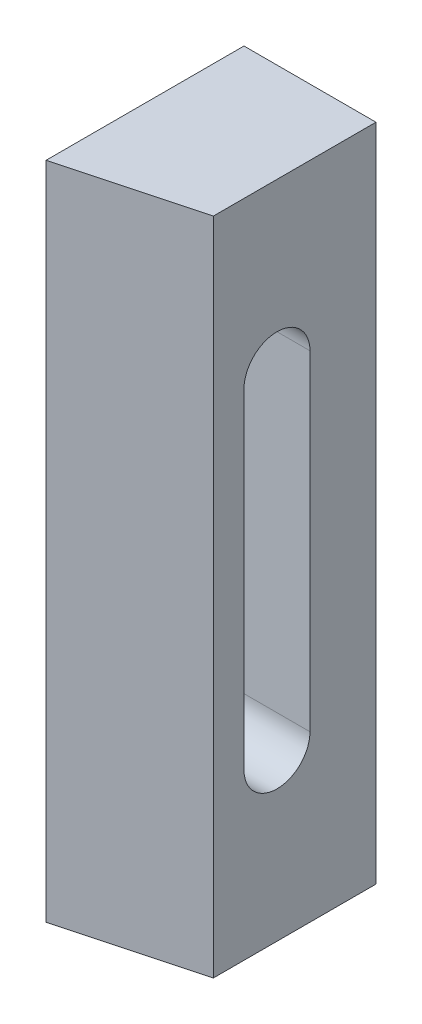
SolidWorks part; units mm, degrees
material "Q235-A"
ref_plane "Front Plane" through (0, 0, 0) normal (0, 0, 1) x (1, 0, 0)
ref_plane "Top Plane" through (0, 0, 0) normal (0, 1, 0) x (1, 0, 0)
ref_plane "Right Plane" through (0, 0, 0) normal (1, 0, 0) x (0, 0, -1)
sketch "Sketch1" plane through (0, 0, 0) normal (1, 0, 0) x (0, 0, -1)
  line L0 (0, 0) -> (60, 0)
  line L1 (60, 0) -> (60, 200)
  line L2 (60, 200) -> (0, 200)
  line L3 (0, 200) -> (0, 0)
  line L4 (30, 50) -> (30, 150) construction
  line L5 (20, 50) -> (20, 150)
  line L6 (40, 50) -> (40, 150)
  arc A0 (20, 50) -> (40, 50) centre (30, 50) ccw
  arc A1 (40, 150) -> (20, 150) centre (30, 150) ccw
  point P8 (30, 100)
  dimension "D4" = 10
  dimension "D5" = 50
  dimension "D6" = 100
  dimension "D8" = 30
  dimension "D1" = 60
  dimension "D2" = 200
extrude "Boss-Extrude1" add sketch "Sketch1" along normal mid plane 40
sketch "Sketch3" plane through (0, 0, 0) normal (0, -1, 0) x (1, 0, 0)
  line L0 (-20, 0) -> (20, -10.718)
  line L1 (20, 0) -> (20, -60) construction
  line L2 (20, -10.718) -> (20, 0)
  line L3 (20, 0) -> (-20, 0)
  line L4 (-20, 0) -> (-20, -60) construction
  dimension "D1" = 75
extrude "Cut-Extrude1" cut sketch "Sketch3" against normal through all
